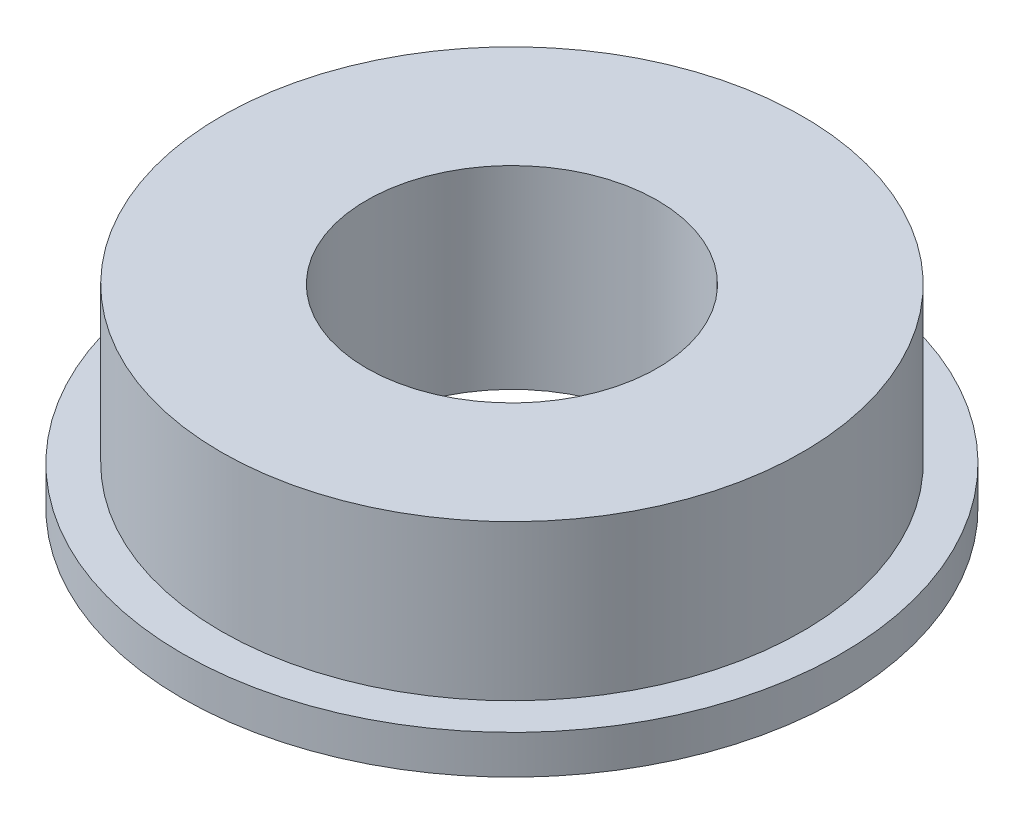
from build123d import *

# Parameters (mm, degrees)
SKETCH_1_R      = 6.8
SKETCH_1_R_2    = 3
EXTRUDE_1_DEPTH = 0.8
SKETCH_2_R      = 6
SKETCH_2_R_2    = 3
EXTRUDE_2_DEPTH = 3.2


with BuildPart() as part:
    # 草图1 → 凸台-拉伸1 (new body)
    with BuildSketch(Plane(origin=(0, 0, 0), x_dir=(1, 0, 0), z_dir=(0, 1, 0))):
        with Locations(Location((0, 0, 0), (0, 0, 270))):
            Circle(SKETCH_1_R)
        with Locations(Location((0, 0, 0), (0, 0, 270))):
            Circle(SKETCH_1_R_2, mode=Mode.SUBTRACT)
    extrude(amount=EXTRUDE_1_DEPTH)

    # 草图2 → 凸台-拉伸2 (add)
    with BuildSketch(Plane(origin=(0, 0.8, 0), x_dir=(1, 0, 0), z_dir=(0, 1, 0))):
        with Locations(Location((0, 0, 0), (0, 0, 270))):
            Circle(SKETCH_2_R)
        with Locations(Location((0, 0, 0), (0, 0, 270))):
            Circle(SKETCH_2_R_2, mode=Mode.SUBTRACT)
    extrude(amount=EXTRUDE_2_DEPTH)


solid = part.part
